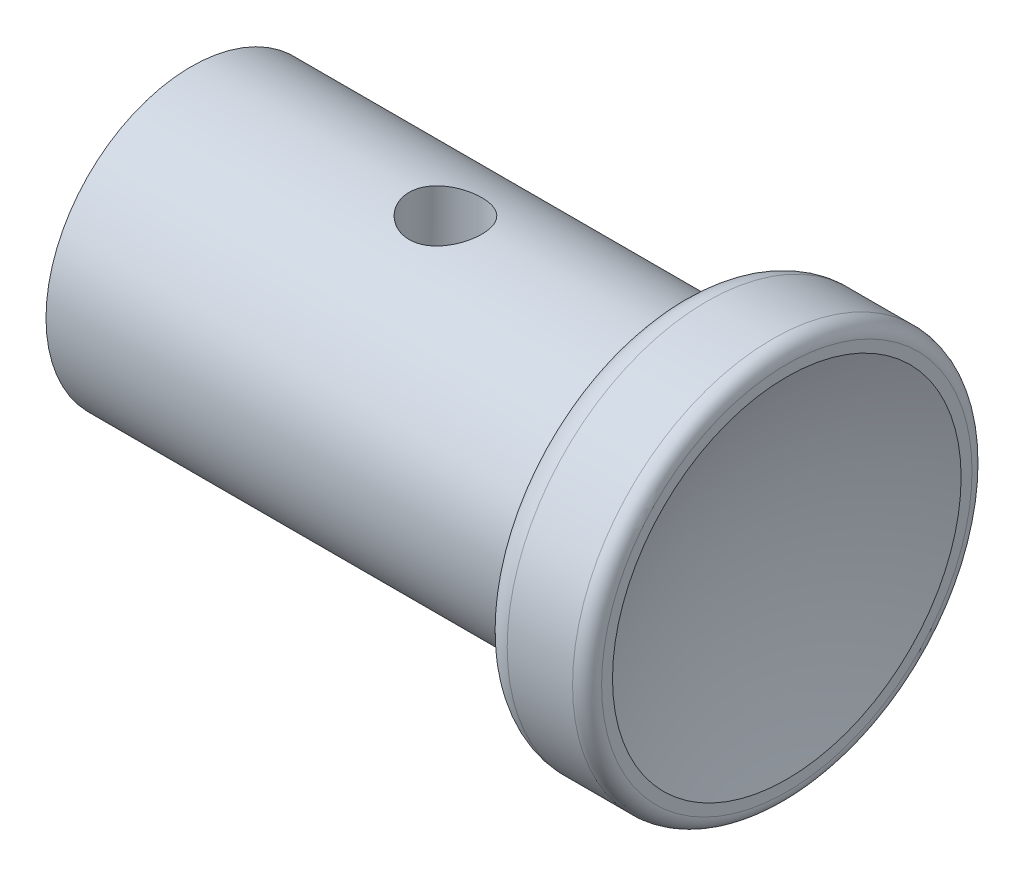
SolidWorks part; units mm, degrees
ref_plane "Front Plane" through (0, 0, 0) normal (0, 0, 1) x (1, 0, 0)
ref_plane "Top Plane" through (0, 0, 0) normal (0, 1, 0) x (1, 0, 0)
ref_plane "Right Plane" through (0, 0, 0) normal (1, 0, 0) x (0, 0, -1)
sketch "Sketch1" plane through (0, 0, 0) normal (0, 0, 1) x (1, 0, 0)
  line L0 (0, 0) -> (145.0892, 0) construction
  line L1 (67, 27.5) -> (67, 20)
  line L2 (0, 0) -> (77.5892, 0)
  line L3 (0, 0) -> (0, 20)
  line L4 (67, 27.5) -> (82, 27.5)
  line L5 (82, 24) -> (82, 27.5)
  line L6 (0, 20) -> (67, 20)
  arc A0 (82, 24) -> (77.5892, 0) centre (145.0892, 0) ccw
  dimension "D6" = 82
  dimension "D1" = 67.5
  dimension "D2" = 40
  dimension "D3" = 55
  dimension "D4" = 67
  dimension "D5" = 3.5
revolve "Revolve1" add sketch "Sketch1" angle 360 about L0
hole_wizard "M24 Tapped Hole1" positions "Sketch3" profile "Sketch2" tap size "M24" standard "GB"
sketch "Sketch3" plane through (0, 0, 0) normal (-1, 0, 0) x (0, 0, 1)
  point P0 (0, 0)
sketch "Sketch2" plane through (0, 0, 0) normal (0, 1, 0) x (0, 0, 1)
  line L0 (0, 0) -> (0, 63.309)
  line L1 (0, 63.309) -> (10.5, 57)
  line L2 (10.5, 57) -> (10.5, 0)
  line L5 (10.5, 0) -> (0, 0)
  line L10 (0, 63.309) -> (-10.5, 57) construction
  line L11 (0, -6.35) -> (0, 107.95) construction
  dimension "螺纹孔钻头直径" = 21
  dimension "螺纹孔钻头深度" = 57
  dimension "导头角度" = 118
cosmetic thread "Cosmetic Thread1" parameters "D1"=48, "D2"=24
sketch "Sketch4" plane through (0, 0, 0) normal (0, 1, 0) x (1, 0, 0)
  line L0 (0, 20) -> (0, -20) construction
  circle A0 centre (35, 0) radius 5
  dimension "D1" = 10
  dimension "D2" = 35
extrude "Cut-Extrude1" cut sketch "Sketch4" against normal mid plane 50
fillet "Fillet2" radius 2 1 edges at (82, 0, 27.5)
fillet "Fillet3" radius 4 1 edges at (67, 0, 27.5)
